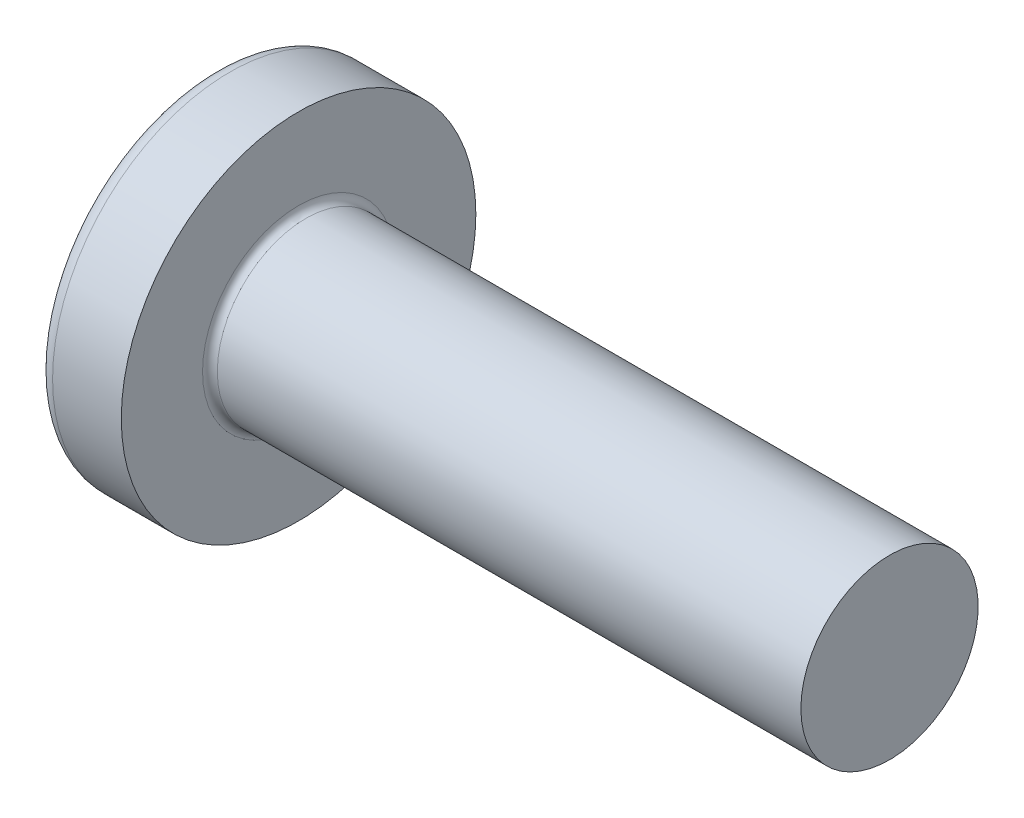
SolidWorks part; units mm, degrees
ref_plane "Front Plane" through (0, 0, 0) normal (0, 0, 1) x (1, 0, 0)
ref_plane "Top Plane" through (0, 0, 0) normal (0, 1, 0) x (1, 0, 0)
ref_plane "Right Plane" through (0, 0, 0) normal (1, 0, 0) x (0, 0, -1)
other "Configuration Table"
sketch "BodySke" plane through (0, 0, 0) normal (0, 0, 1) x (1, 0, 0)
  line L0 (0, 0) -> (156.4409, 0) construction
  line L1 (0, 0) -> (0, 48.4317) construction
  line L2 (0, 0) -> (24.6, 0)
  line L3 (24.6, 0) -> (24.6, 3)
  line L4 (24.6, 3) -> (4.6, 3)
  line L5 (4.6, 3) -> (4.6, 6)
  line L6 (4.6, 6) -> (2.2747, 6)
  line L7 (5.6, 0) -> (5.6, 8.4138) construction
  line L8 (4.6, 0) -> (4.6, 8.4138) construction
  arc A0 (0, 0) -> (1.8337, 5.7717) centre (10, 0) cw
  arc A1 (2.2747, 6) -> (1.8337, 5.7717) centre (2.2747, 5.46) ccw
  point P14 (24.6, 2.4455)
revolve "BaseBody" add sketch "BodySke" angle 360 about L0
cosmetic thread "ThreadCosmetic" [suppressed] parameters "Thread_length"=20, "Thread_minor"=4.891
fillet "Fillet1" radius 0.25 1 edges at (4.6, 0, 3)
ref_plane "Plane1" through (3.46, 0, 0) normal (1, 0, 0) x (0, 0, -1)
sketch "RecessTopSke" plane through (0, 0, 0) normal (1, 0, 0) x (0, 0, -1)
  line L0 (-0.71, 3.35) -> (0.71, -3.35) construction
  line L1 (-0.71, 3.35) -> (0.71, 3.35)
  line L2 (-0.71, 3.35) -> (-0.71, -3.35)
  line L3 (-0.71, -3.35) -> (0.71, -3.35)
  line L4 (0.71, 3.35) -> (0.71, -3.35)
sketch "RecessBottomSke" plane through (3.46, 0, 0) normal (1, 0, 0) x (0, 0, -1)
  line L0 (-0.71, 3.35) -> (-0.71, -3.35) construction
  line L1 (-0.71, -1.4405) -> (0.71, -1.4405)
  line L2 (-0.71, -1.4405) -> (-0.71, 1.4405)
  line L3 (-0.71, 1.4405) -> (0.71, 1.4405)
  line L4 (0.71, -1.4405) -> (0.71, 1.4405)
  line L5 (0.71, 3.35) -> (0.71, -3.35) construction
  line L6 (-0.71, -1.4405) -> (0.71, 1.4405) construction
loft "Recess" cut profiles "RecessTopSke", "RecessBottomSke"
pattern_circular "RecPat" count 2 over 90 about axis through (0, 0, 0) along (1, 0, 0) of "Recess"
sketch "RecessCoreSke" plane through (0, 0, 0) normal (0, 0, 1) x (1, 0, 0)
  line L0 (0, 0) -> (51.8769, 0) construction
  line L1 (0, 0) -> (3.8761, 0)
  line L2 (3.8761, 0) -> (3.46, 1.2805)
  line L3 (3.46, 1.2805) -> (0, 1.5224)
  line L4 (0, 1.5224) -> (0, 0)
revolve "RecessCore" cut sketch "RecessCoreSke" angle 360 about L0
sketch "ThdSchSke" plane through (0, 0, 0) normal (0, 0, 1) x (1, 0, 0)
  line L0 (0, 0) -> (54.2585, 0) construction
  line L1 (24.2799, 3.6403) -> (24.2799, 3)
  line L2 (24.2799, 3.6403) -> (24.9201, 3.6403)
  line L3 (24.9201, 3.6403) -> (24.9201, 3)
  line L4 (24.9201, 3) -> (24.6, 2.4455)
  line L5 (24.6, 2.4455) -> (24.2799, 3)
  line L6 (24.6, 3) -> (4.6, 3) construction
revolve "ThreadSchematic" [suppressed] cut sketch "ThdSchSke" angle 360 about L0
pattern_linear "ThdSchPat" [suppressed]
equation "\"Thread_minor@ThreadCosmetic\" = \"Thread_minor@BodySke\""
equation "\"Thread_length@ThreadCosmetic\" = \"Thread_length@BodySke\""
equation "\"D1@RecessBottomSke\" = \"Cross_diameter@RecessTopSke\"  * 0.43"
equation "\"D1@RecessCoreSke\" = \"Cross_depth@Plane1\""
equation "\"Tooth_Num@ThdSchPat\" =  int( \"Thread_length@BodySke\" / \"Advance@BodySke\" ) "
equation "\"Advance@ThdSchPat\" = \"Advance@BodySke\""
